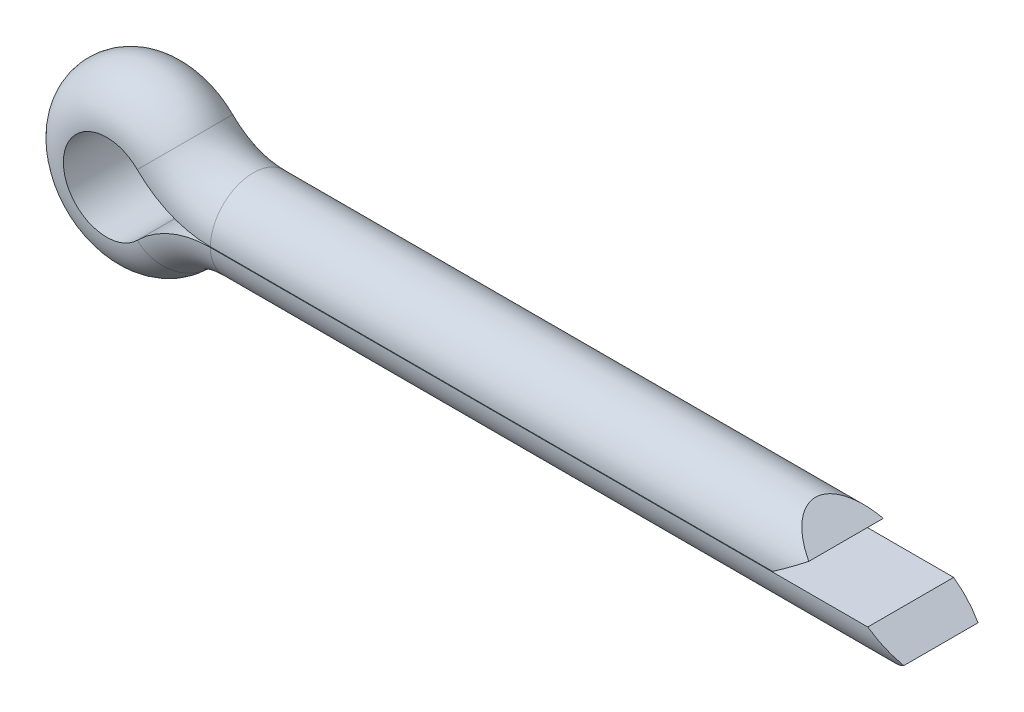
SolidWorks part; units mm, degrees
ref_plane "Front Plane" through (0, 0, 0) normal (0, 0, 1) x (1, 0, 0)
ref_plane "Top Plane" through (0, 0, 0) normal (0, 1, 0) x (1, 0, 0)
ref_plane "Right Plane" through (0, 0, 0) normal (1, 0, 0) x (0, 0, -1)
sketch "Dimension sketch" plane through (0, 0, 0) normal (0, 0, 1) x (1, 0, 0)
  line L0 (23.5, 1.45) -> (3.5, 1.45)
  line L1 (3.5, -1.45) -> (26.7, -1.45)
  line L2 (3.5, 0) -> (27.3859, 0) construction
  line L3 (3.5, 0) -> (3.5, -0.0723) construction
  line L4 (-2.9, 0) -> (-2.9, 18.8979) construction
  arc A0 (3.5, 1.45) -> (2.0509, 2.0504) centre (3.5, 3.4991) cw
  arc A1 (2.0509, 2.0504) -> (2.0509, -2.0504) centre (0, 0) ccw
  arc A2 (2.0509, -2.0504) -> (3.5, -1.45) centre (3.5, -3.4991) cw
  dimension "c" = 5.8
  dimension "d1" = 2.9
  dimension "b" = 6.4
  dimension "l" = 20
  dimension "a" = 3.2
ref_plane "Plane1" through (23.5, 1.45, 0) normal (-1, 0, 0) x (0, 0, 1)
sketch "Sketch2" plane through (23.5, 1.45, 0) normal (-1, 0, 0) x (0, 0, 1)
  line L0 (0, -4.35) -> (0, 1.45) construction
  line L1 (-1.45, -1.44) -> (1.45, -1.44)
  arc A0 (1.45, -1.44) -> (-1.45, -1.44) centre (0, -1.45) ccw
  dimension "d" = 2.9
  dimension "D1" = 0.01
sweep "Sweep2" add profiles "Sketch2" path "Dimension sketch"
sketch "Sketch3" plane through (0, 0, 0) normal (0, 0, 1) x (1, 0, 0)
  line L0 (3.5, 0) -> (3.5, 16.2682) construction
  line L1 (3.5, 0) -> (37.4999, 0) construction
  line L2 (26.7, -1.45) -> (26.7, -0.01) construction
  line L3 (23.5, 0.72) -> (22.4681, 1.45)
  line L4 (23.5, 1.45) -> (3.5, 1.45) construction
  line L5 (3.5, -1.45) -> (26.7, -1.45) construction
  line L6 (23.5, 0.72) -> (22.4611, 0)
  line L7 (26.7, -0.73) -> (25.6681, 0)
  line L9 (26.7, -0.73) -> (25.6611, -1.45)
  line L10 (25.6681, 0) -> (22.4611, 0)
  line L11 (22.4681, 1.45) -> (26.71, 1.45)
  line L12 (26.71, 1.45) -> (26.71, -1.45)
  line L13 (26.71, -1.45) -> (25.6611, -1.45)
  line L14 (23.5, 1.45) -> (23.5, 0.01) construction
  dimension "D1" = 0.01
  dimension "D3" = 70
  dimension "D4" = 70
extrude "Cut-Extrude1" cut sketch "Sketch3" against normal through all and the other way through all
